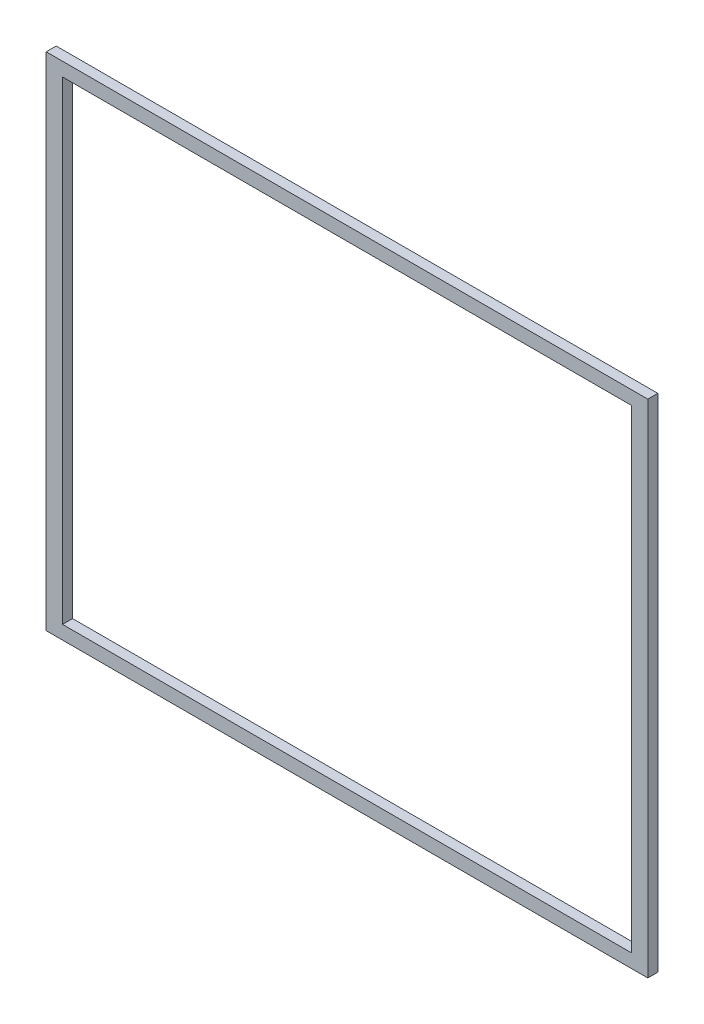
from build123d import *

# Parameters (mm, degrees)
SKETCH1_W           = 600
SKETCH1_H           = 500
SKETCH1_W_2         = 567.390239782
SKETCH1_H_2         = 472.825199818
BOSS_EXTRUDE1_DEPTH = 10


with BuildPart() as part:
    # Sketch1 → Boss-Extrude1 (new body)
    with BuildSketch(Plane.XY):
        Rectangle(SKETCH1_W, SKETCH1_H)
        Rectangle(SKETCH1_W_2, SKETCH1_H_2, mode=Mode.SUBTRACT)
    extrude(amount=BOSS_EXTRUDE1_DEPTH)


solid = part.part
